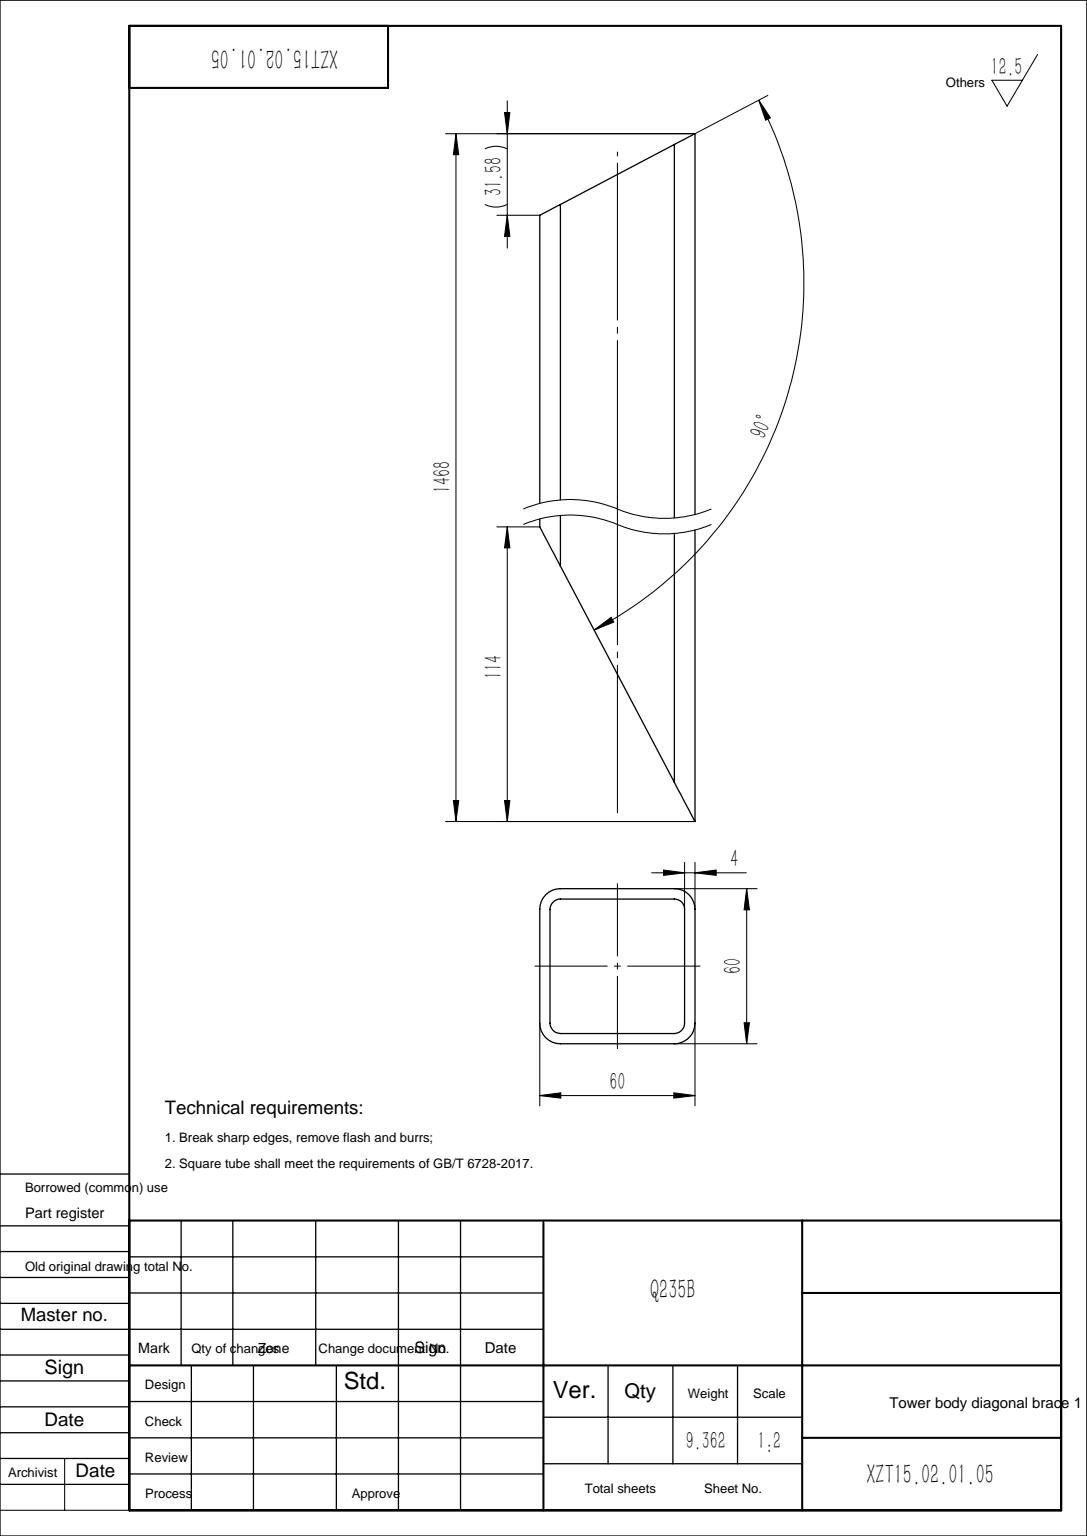
SolidWorks part; units mm, degrees
material "Q235B"
ref_plane "Front Plane" through (0, 0, 0) normal (0, 0, 1) x (1, 0, 0)
ref_plane "Top Plane" through (0, 0, 0) normal (0, 1, 0) x (1, 0, 0)
ref_plane "Right Plane" through (0, 0, 0) normal (1, 0, 0) x (0, 0, -1)
sketch "草图1" plane through (0, 0, 0) normal (0, 0, 1) x (1, 0, 0)
  line L0 (0, 0) -> (0, 1468)
  dimension "D1" = 1468
other "GB/T 6728-2002 square hollow section 60×60×4(1)"
ref_plane "Plane1" through (0, 0, 0) normal (0, 1, 0) x (-1, 0, 0)
sketch "Sketch1" plane through (0, 0, 0) normal (0, 1, 0) x (-1, 0, 0)
  line L0 (-22, -26) -> (22, -26)
  line L1 (-26, -22) -> (-26, 22)
  line L2 (22, 26) -> (-22, 26)
  line L3 (26, 22) -> (26, -22)
  line L4 (-22, -30) -> (22, -30)
  line L5 (-30, -22) -> (-30, 22)
  line L6 (22, 30) -> (-22, 30)
  line L7 (30, 22) -> (30, -22)
  arc A0 (30, 22) -> (22, 30) centre (22, 22) ccw
  arc A1 (22, -30) -> (30, -22) centre (22, -22) ccw
  arc A2 (-30, -22) -> (-22, -30) centre (-22, -22) ccw
  arc A3 (-22, 30) -> (-30, 22) centre (-22, 22) ccw
  arc A4 (-22, 26) -> (-26, 22) centre (-22, 22) ccw
  arc A5 (26, 22) -> (22, 26) centre (22, 22) ccw
  arc A6 (22, -26) -> (26, -22) centre (22, -22) ccw
  arc A7 (-26, -22) -> (-22, -26) centre (-22, -22) ccw
  point P0 (-30, 0)
  point P1 (30, 0)
  point P2 (0, 30)
  point P3 (0, -30)
  point P4 (0, 0)
  point P5 (-30, -30)
  point P6 (30, -30)
  point P7 (30, 30)
  point P8 (-30, 30)
  point P33 (0, 0)
  dimension "D1" = 8
  dimension "Thickness" = 4
  dimension "V_leg" = 60
sketch "Sketch2" plane through (0, 0, 30) normal (0, 0, 1) x (1, 0, 0)
  line L4 (-30, 0) -> (-30, 114)
  line L5 (-30, 1468) -> (-30, 0) construction
  line L6 (-30, 114) -> (30, 0)
  line L7 (30, 0) -> (-30, 0)
  line L9 (-30, 1436.4211) -> (30, 1468)
  line L10 (30, 1468) -> (-30, 1468)
  line L11 (-30, 1468) -> (-30, 1436.4211)
  dimension "D1" = 114
  dimension "D2" = 90
  dimension "D3" = 31.5789
extrude "Cut-Extrude1" cut sketch "Sketch2" against normal through all both and the other way through all
